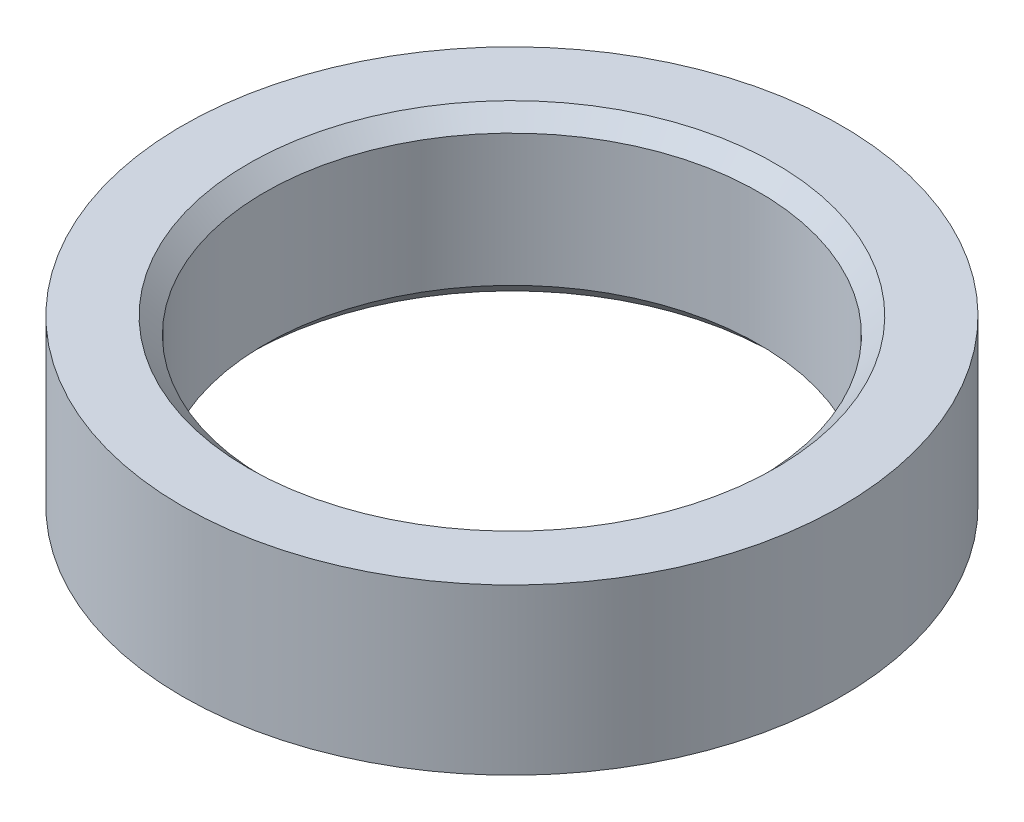
from build123d import *

# Parameters (mm, degrees)
SKETCH_1_R          = 4
SKETCH_1_R_2        = 3
EXTRUDE_1_DEPTH     = 2
CHAMFER_C0_2_1_SIZE = 0.2


with BuildPart() as part:
    # 草图1 → 凸台-拉伸1 (new body)
    with BuildSketch(Plane(origin=(0, 0, 0), x_dir=(1, 0, 0), z_dir=(0, 1, 0))):
        with Locations(Location((0, 0, 0), (0, 0, 270))):
            Circle(SKETCH_1_R)
        with Locations(Location((0, 0, 0), (0, 0, 270))):
            Circle(SKETCH_1_R_2, mode=Mode.SUBTRACT)
    extrude(amount=EXTRUDE_1_DEPTH)

    # C0.2 倒角1
    chamfer_c0_2_1_edges = [part.edges().sort_by_distance(p)[0] for p in [
        (0, 0, -3),
        (0, 2, -3),
    ]]
    chamfer(chamfer_c0_2_1_edges, length=CHAMFER_C0_2_1_SIZE)


solid = part.part
